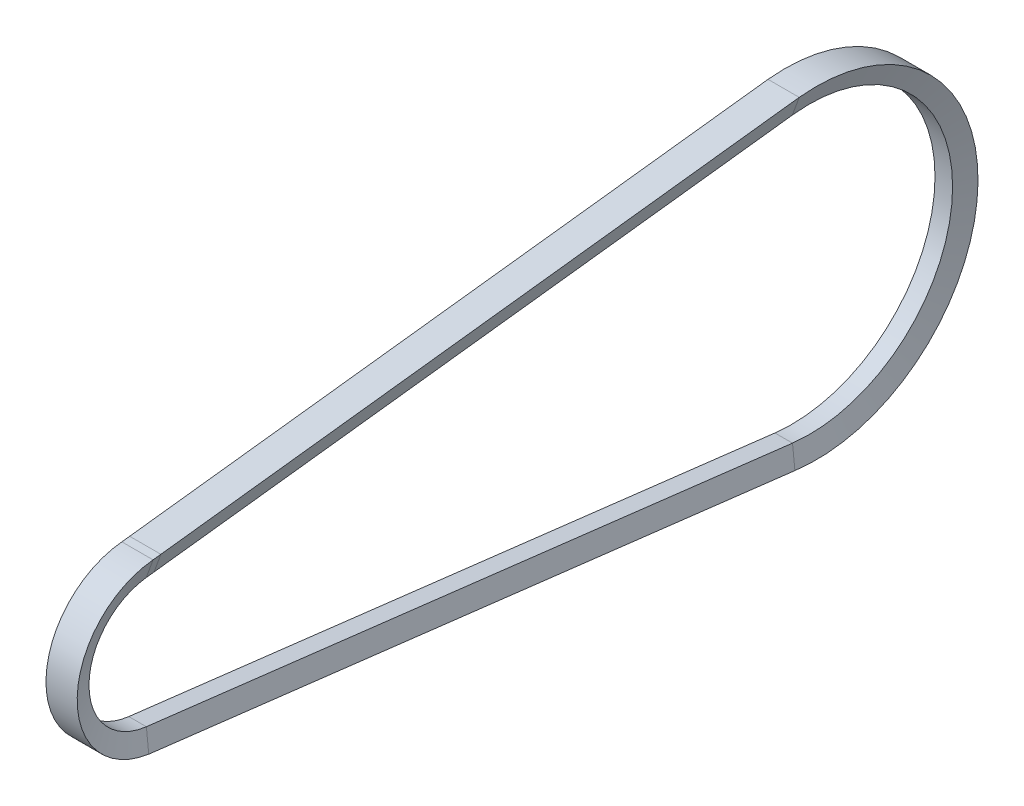
SolidWorks part; units mm, degrees
ref_plane "Front Plane" through (0, 0, 0) normal (0, 0, 1) x (1, 0, 0)
ref_plane "Top Plane" through (0, 0, 0) normal (0, 1, 0) x (1, 0, 0)
ref_plane "Right Plane" through (0, 0, 0) normal (1, 0, 0) x (0, 0, -1)
other "Configuration Table"
sketch "Sketch2" plane through (0, 0, 0) normal (0, 0, 1) x (1, 0, 0)
  line L7 (-5, 6) -> (5, 6)
  line L8 (0, 6.6921) -> (0, -6.2165) construction
  line L9 (5, 6) -> (2.8162, 0)
  line L10 (-2.8162, 0) -> (2.8162, 0)
  line L11 (-5, 6) -> (-2.8162, 0)
  point P3 (0, 0)
  point P11 (0, 6)
  dimension "D1" = 10
  dimension "D2" = 6
  dimension "D3" = 40
sketch "Sketch3" plane through (0, 0, 0) normal (1, 0, 0) x (0, 0, -1)
  line L0 (0, 6.6921) -> (0, -6.2165) construction
  line L1 (0, -21) -> (210, -21) construction
  line L2 (-2.5, -0.1493) -> (204.5238, 24.6729)
  line L3 (-2.5, -41.8507) -> (204.5238, -66.6729)
  arc A0 (-2.5, -0.1493) -> (-2.5, -41.8507) centre (0, -21) ccw
  arc A1 (204.5238, -66.6729) -> (204.5238, 24.6729) centre (210, -21) ccw
  dimension "D1" = 92
  dimension "D3" = 42
  dimension "D2" = 210
sweep "Sweep1" add profiles "Sketch2" path "Sketch3"
